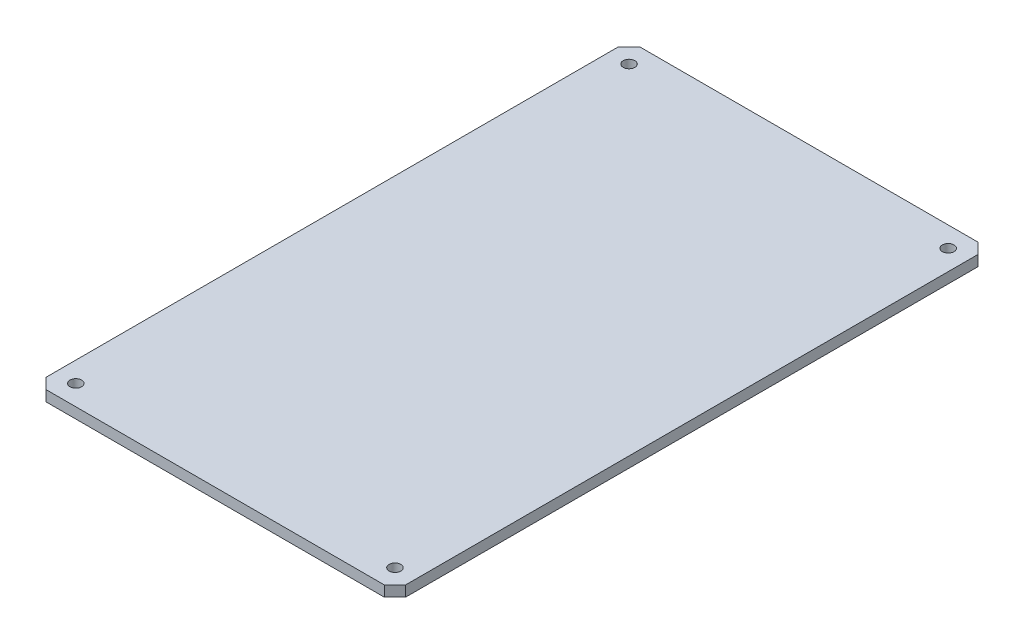
SolidWorks part; units mm, degrees
material "6061"
ref_plane "前视基准面" through (0, 0, 0) normal (0, 0, 1) x (1, 0, 0)
ref_plane "上视基准面" through (0, 0, 0) normal (0, 1, 0) x (1, 0, 0)
ref_plane "右视基准面" through (0, 0, 0) normal (1, 0, 0) x (0, 0, -1)
sketch "草图1" plane through (0, 0, 0) normal (0, 1, 0) x (1, 0, 0)
  line L1 (84.5, -139.5) -> (-84.5, -139.5)
  line L2 (84.5, -139.5) -> (84.5, 139.5)
  line L3 (84.5, 139.5) -> (-84.5, 139.5)
  line L4 (-84.5, -139.5) -> (-84.5, 139.5)
  line L5 (84.5, -139.5) -> (-84.5, 139.5) construction
  line L6 (84.5, 139.5) -> (-84.5, -139.5) construction
  point P0 (0, 0)
  dimension "D1" = 169
  dimension "D2" = 279
extrude "凸台-拉伸1" add sketch "草图1" along normal mid plane 5
hole_wizard "Ø5.5 (5.5) 直径孔1" positions "草图2" profile "草图3" hole size "Ø5.5" standard "GB" end condition through all
sketch "草图2" plane through (0, -2.5, 0) normal (0, -1, 0) x (-1, 0, 0)
  line L1 (75, -130) -> (-75, -130)
  line L2 (75, -130) -> (75, 130)
  line L3 (75, 130) -> (-75, 130)
  line L4 (-75, -130) -> (-75, 130)
  line L5 (75, -130) -> (-75, 130)
  point P0 (75, -130)
  point P2 (-75, -130)
  point P4 (-75, 130)
  point P6 (75, 130)
  dimension "D1" = 260
  dimension "D2" = 150
sketch "草图3" plane through (-75, -2.5, 130) normal (1, 0, 0) x (0, 0, -1)
  line L0 (0, 0) -> (0, 5)
  line L1 (0, 5) -> (2.75, 5)
  line L2 (2.75, 5) -> (2.75, 0)
  line L5 (2.75, 0) -> (0, 0)
  line L11 (0, -6.35) -> (0, 107.95) construction
  dimension "通孔孔直径" = 5.5
  dimension "通孔孔深度" = 5
chamfer "倒角1" distance 5 angle 45 4 edges at (84.5, 0, -139.5) (-84.5, 0, -139.5) (84.5, 0, 139.5) (-84.5, 0, 139.5)
